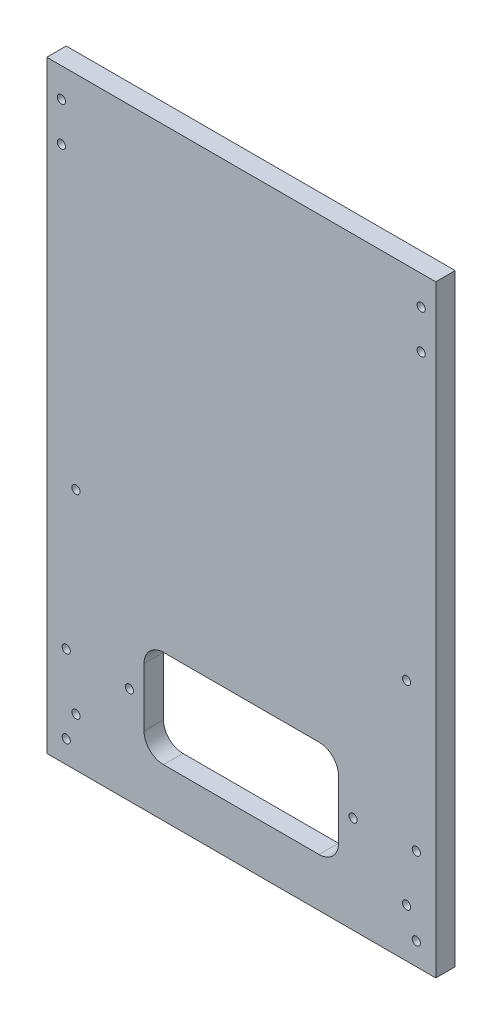
from build123d import *

# Parameters (mm, degrees)
SKETCH_1_W          = 200
SKETCH_1_H          = 310
EXTRUDE_1_DEPTH     = 5
SKETCH_2_W          = 100
SKETCH_2_H          = 50
CUT_EXTRUDE_1_DEPTH = 185.729532019
HOLE_WIZARD_M5_2_D  = 4.2
FILLET_1_R          = 10
HOLE_WIZARD_M5_4_D  = 4.2
HOLE_WIZARD_M5_5_D  = 4.2
HOLE_WIZARD_M5_6_D  = 4.2


with BuildPart() as part:
    # 草图1 → 凸台-拉伸1 (new, symmetric)
    with BuildSketch(Plane.XY):
        Rectangle(SKETCH_1_W, SKETCH_1_H)
    extrude(amount=EXTRUDE_1_DEPTH, both=True)

    # 草图2 → 切除-拉伸1 (cut, through all)
    with BuildSketch(Plane.XY.offset(5)):
        with Locations((0, -105)):
            Rectangle(SKETCH_2_W, SKETCH_2_H)
    extrude(amount=-CUT_EXTRUDE_1_DEPTH, mode=Mode.SUBTRACT)

    # M5 螺纹孔2 (through all)
    with Locations(Plane.XY.offset(5)):
        with Locations((85, -130), (85, -30), (-85, -30), (-85, -130)):
            Hole(HOLE_WIZARD_M5_2_D / 2)

    # 圆角1
    fillet_1_edges = [part.edges().sort_by_distance(p)[0] for p in [
        (50, -80, 0),
        (50, -130, 0),
        (-50, -130, 0),
        (-50, -80, 0),
    ]]
    fillet(fillet_1_edges, radius=FILLET_1_R)

    # M5 螺纹孔4 (through all)
    with Locations(Plane(origin=(0, 0, -5), x_dir=(-1, 0, 0), z_dir=(0, 0, -1))):
        with Locations((92.5, 120), (92.5, 140), (-92.5, 140), (-92.5, 120)):
            Hole(HOLE_WIZARD_M5_4_D / 2)

    # M5 螺纹孔5 (through all)
    with Locations(Plane(origin=(0, 0, -5), x_dir=(-1, 0, 0), z_dir=(0, 0, -1))):
        with Locations((-57.5, -105), (57.5, -105)):
            Hole(HOLE_WIZARD_M5_5_D / 2)

    # M5 螺纹孔6 (through all)
    with Locations(Plane(origin=(0, 0, -5), x_dir=(-1, 0, 0), z_dir=(0, 0, -1))):
        with Locations((90, -143.5), (90, -103.5), (-90, -103.5), (-90, -143.5)):
            Hole(HOLE_WIZARD_M5_6_D / 2)


solid = part.part
